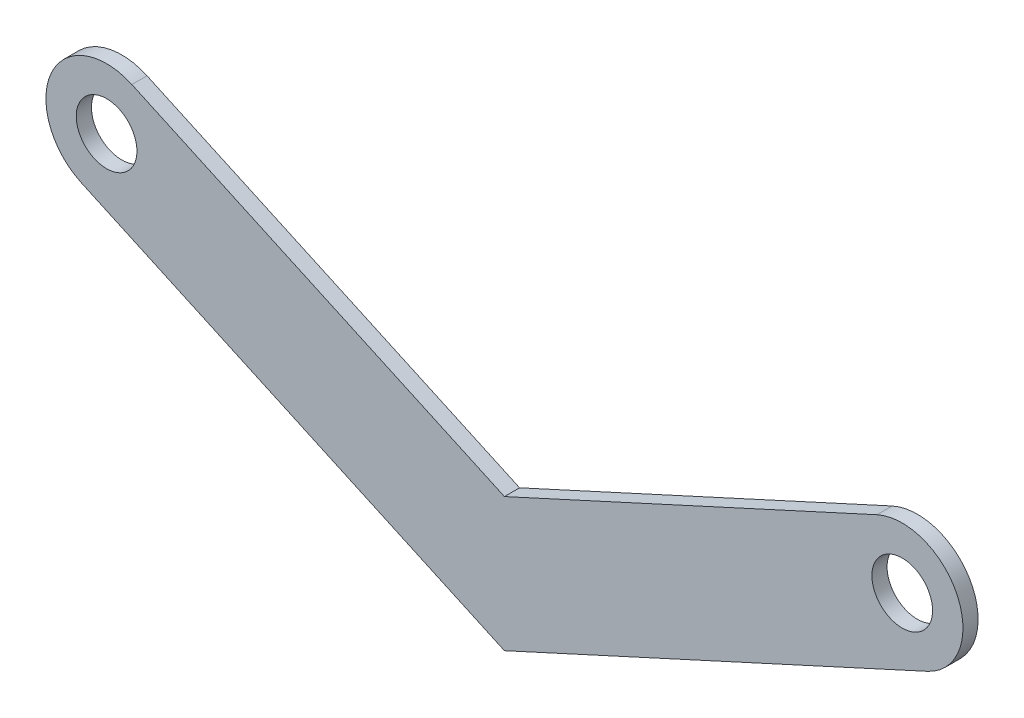
SolidWorks part; units mm, degrees
ref_plane "Front Plane" through (0, 0, 0) normal (0, 0, 1) x (1, 0, 0)
ref_plane "Top Plane" through (0, 0, 0) normal (0, 1, 0) x (1, 0, 0)
ref_plane "Right Plane" through (0, 0, 0) normal (1, 0, 0) x (0, 0, -1)
sketch "Sketch1" plane through (0, 0, 0) normal (0, 0, 1) x (1, 0, 0)
  line L0 (0, 0) -> (0, 98.9014) construction
  line L1 (-63.5177, -61.9319) -> (65.55, 41.002) construction
  line L6 (0, 21.9956) -> (61.388, 50.0947)
  line L13 (0, 0) -> (69.712, 31.9093)
  line L14 (0, 21.9956) -> (-61.388, 50.0947)
  line L15 (0, 0) -> (-69.712, 31.9093)
  arc A8 (69.712, 31.9093) -> (61.388, 50.0947) centre (65.55, 41.002) ccw
  arc A9 (-69.712, 31.9093) -> (-61.388, 50.0947) centre (-65.55, 41.002) cw
  circle A10 centre (-65.55, 41.002) radius 5
  circle A11 centre (65.55, 41.002) radius 5
  point P5 (0, 0)
  dimension "D2" = 131.1
  dimension "D1" = 10
  dimension "D3" = 10
  dimension "D4" = 130.81
  dimension "D5" = 20
extrude "Boss-Extrude1" add sketch "Sketch1" along normal blind 2.5
